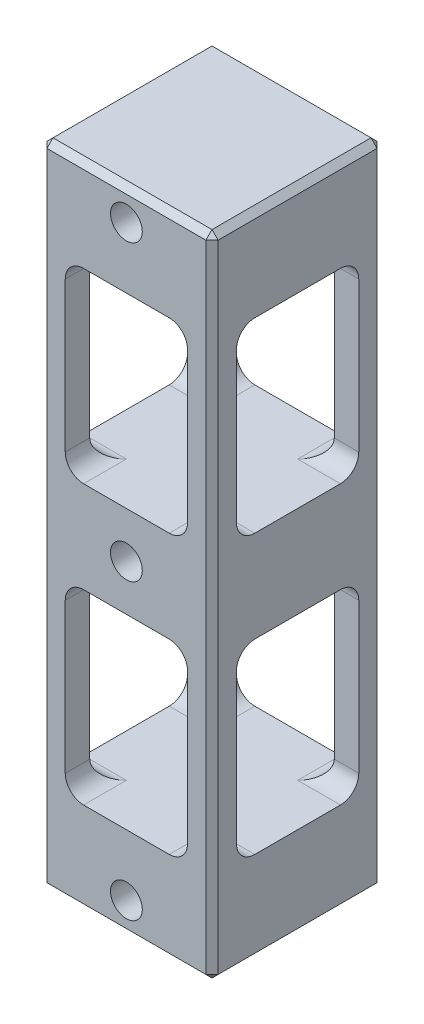
from build123d import *

# Parameters (mm, degrees)
SKETCH_1_W          = 28
SKETCH_1_H          = 28
EXTRUDE_1_DEPTH     = 106
SKETCH_2_R          = 2.6
CUT_EXTRUDE_1_DEPTH = 111.526015037
CUT_EXTRUDE_2_DEPTH = 111.526015037
CHAMFER_1_SIZE      = 1


with BuildPart() as part:
    # 草图1 → 凸台-拉伸1 (new body)
    with BuildSketch(Plane(origin=(0, 0, 0), x_dir=(1, 0, 0), z_dir=(0, 1, 0))):
        Rectangle(SKETCH_1_W, SKETCH_1_H)
    extrude(amount=EXTRUDE_1_DEPTH)

    # 草图2 → 切除-拉伸1 (cut, through all)
    with BuildSketch(Plane.XY.offset(14)):
        with Locations((0, 101)):
            Circle(SKETCH_2_R)
        with Locations((0, 53)):
            Circle(SKETCH_2_R)
        with Locations((0, 5)):
            Circle(SKETCH_2_R)
        with BuildLine():
            Line((-7, 60.5), (7, 60.5))
            ThreePointArc((7, 60.5), (9.121320344, 61.378679656), (10, 63.5))
            Line((10, 63.5), (10, 88))
            ThreePointArc((10, 88), (9.121320344, 90.121320344), (7, 91))
            Line((7, 91), (-7, 91))
            ThreePointArc((-7, 91), (-9.121320344, 90.121320344), (-10, 88))
            Line((-10, 88), (-10, 63.5))
            ThreePointArc((-10, 63.5), (-9.121320344, 61.378679656), (-7, 60.5))
        make_face()
        with BuildLine():
            Line((-7, 15), (7, 15))
            ThreePointArc((7, 15), (9.121320344, 15.878679656), (10, 18))
            Line((10, 18), (10, 42.5))
            ThreePointArc((10, 42.5), (9.121320344, 44.621320344), (7, 45.5))
            Line((7, 45.5), (-7, 45.5))
            ThreePointArc((-7, 45.5), (-9.121320344, 44.621320344), (-10, 42.5))
            Line((-10, 42.5), (-10, 18))
            ThreePointArc((-10, 18), (-9.121320344, 15.878679656), (-7, 15))
        make_face()
    extrude(amount=-CUT_EXTRUDE_1_DEPTH, mode=Mode.SUBTRACT)

    # 草图3 → 切除-拉伸2 (cut, through all)
    with BuildSketch(Plane(origin=(14, 0, 0), x_dir=(0, 0, -1), z_dir=(1, 0, 0))):
        with BuildLine():
            Line((-7, 60.5), (7, 60.5))
            ThreePointArc((7, 60.5), (9.121320344, 61.378679656), (10, 63.5))
            Line((10, 63.5), (10, 88))
            ThreePointArc((10, 88), (9.121320344, 90.121320344), (7, 91))
            Line((7, 91), (-7, 91))
            ThreePointArc((-7, 91), (-9.121320344, 90.121320344), (-10, 88))
            Line((-10, 88), (-10, 63.5))
            ThreePointArc((-10, 63.5), (-9.121320344, 61.378679656), (-7, 60.5))
        make_face()
        with BuildLine():
            Line((-7, 15), (7, 15))
            ThreePointArc((7, 15), (9.121320344, 15.878679656), (10, 18))
            Line((10, 18), (10, 42.5))
            ThreePointArc((10, 42.5), (9.121320344, 44.621320344), (7, 45.5))
            Line((7, 45.5), (-7, 45.5))
            ThreePointArc((-7, 45.5), (-9.121320344, 44.621320344), (-10, 42.5))
            Line((-10, 42.5), (-10, 18))
            ThreePointArc((-10, 18), (-9.121320344, 15.878679656), (-7, 15))
        make_face()
    extrude(amount=-CUT_EXTRUDE_2_DEPTH, mode=Mode.SUBTRACT)

    # 倒角1
    chamfer_1_edges = [part.edges().sort_by_distance(p)[0] for p in [
        (-14, 106, 0),
        (0, 106, 14),
        (14, 106, 0),
        (0, 0, 14),
        (-14, 0, 0),
        (0, 0, -14),
        (14, 0, 0),
        (14, 53, 14),
        (-14, 53, 14),
        (-14, 53, -14),
        (14, 53, -14),
        (0, 106, -14),
    ]]
    chamfer(chamfer_1_edges, length=CHAMFER_1_SIZE)


solid = part.part
